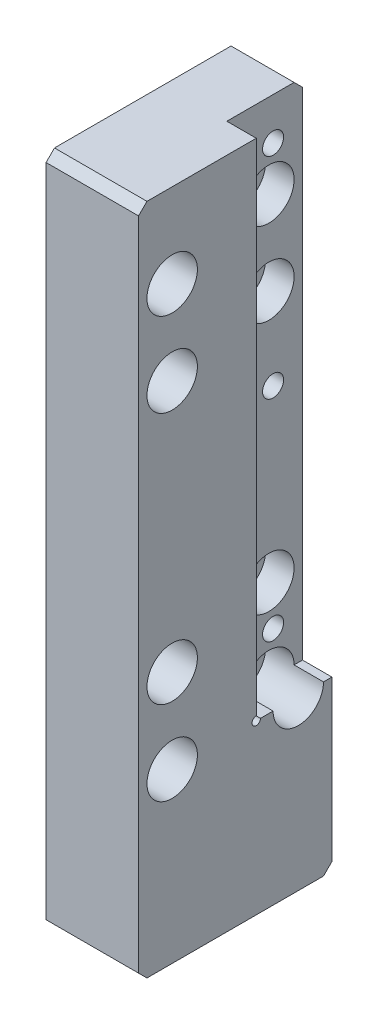
SolidWorks part; units mm, degrees
material "45#"
ref_plane "前基準面" through (0, 0, 0) normal (0, 0, 1) x (1, 0, 0)
ref_plane "上基準面" through (0, 0, 0) normal (0, 1, 0) x (1, 0, 0)
ref_plane "右基準面" through (0, 0, 0) normal (1, 0, 0) x (0, 0, -1)
sketch "草图1" plane through (0, 0, 0) normal (0, 1, 0) x (1, 0, 0)
  line L0 (0, 0) -> (0, 23)
  line L1 (0, 23) -> (11, 23)
  line L4 (11, 23) -> (11, 0)
  line L5 (11, 0) -> (0, 0)
  dimension "D2" = 11
  dimension "D3" = 23
extrude "凸台-拉伸1" add sketch "草图1" along normal blind 80
sketch "草图2" plane through (11, 0, 0) normal (1, 0, 0) x (0, 0, -1)
  line L1 (23, 80) -> (14, 80)
  line L2 (23, 80) -> (23, 20)
  line L3 (23, 20) -> (14.5, 20)
  line L4 (14, 80) -> (14, 20.5)
  arc A0 (14, 20.5) -> (14.5, 20) centre (14, 20) ccw
  dimension "D3" = 1
  dimension "D1" = 60
  dimension "D2" = 9
extrude "切除-拉伸1" cut sketch "草图2" against normal blind 3.5
hole_wizard "打孔尺寸(%根据)内六角圆柱头螺钉的类型2" positions "草图3" profile "草图4" counterbore size "M3" standard "GB" end condition through all
sketch "草图3" plane through (11, 0, 0) normal (1, 0, 0) x (0, 0, -1)
  line L0 (11.5, 0) -> (11.5, 103.8051) construction
  line L1 (0, 0) -> (23, 0) construction
  point P0 (4, 20)
  point P2 (4, 30)
  point P14 (19, 30)
  point P15 (19, 20)
  point P20 (4, 60)
  point P21 (4, 70)
  point P25 (19, 60) [skipped]
  point P26 (19, 70) [skipped]
  point P27 (19, 70)
  point P28 (19, 60)
  dimension "D1" = 15
  dimension "D2" = 20
  dimension "D3" = 10
  dimension "D5" = 40
  dimension "D4" = 2
sketch "草图4" plane through (11, 20, -4) normal (0, 1, 0) x (0, 0, -1)
  line L0 (0, 0) -> (0, 11)
  line L1 (0, 11) -> (1.7, 11)
  line L3 (1.7, 11) -> (1.7, 6.9)
  line L4 (1.7, 6.9) -> (3, 6.9)
  line L5 (3, 6.9) -> (3, 0)
  line L7 (3, 0) -> (0, 0)
  line L11 (0, -6.35) -> (0, 107.95) construction
  dimension "通孔孔直径" = 3.4
  dimension "通孔孔深度" = 11
  dimension "柱形沉头孔直径" = 6
  dimension "柱形沉头孔深度" = 6.9
hole_wizard "M5 螺纹孔1" positions "草图5" profile "草图6" tap size "M5" standard "GB"
sketch "草图5" plane through (0, 0, 0) normal (0, -1, 0) x (-1, 0, 0)
  line L4 (0, 11.5) -> (-11, 11.5) construction
  line L5 (0, 23) -> (0, 0) construction
  line L6 (-11, 0) -> (-11, 23) construction
  point P0 (-5.5, 11.5)
sketch "草图6" plane through (5.5, 0, -11.5) normal (1, 0, 0) x (0, 0, -1)
  line L0 (0, 0) -> (0, 13.6618)
  line L1 (0, 13.6618) -> (2.1, 12.4)
  line L2 (2.1, 12.4) -> (2.1, 0)
  line L5 (2.1, 0) -> (0, 0)
  line L10 (0, 13.6618) -> (-2.1, 12.4) construction
  line L11 (0, -6.35) -> (0, 107.95) construction
  dimension "螺纹孔钻头直径" = 4.2
  dimension "螺纹孔钻头深度" = 12.4
  dimension "导头角度" = 118
cosmetic thread "孔螺蚊线1" parameters "D1"=10, "D2"=5
hole_wizard "M3 螺纹孔1" positions "草图9" profile "草图10" tap size "M3" standard "GB" end condition through all
sketch "草图9" plane through (7.5, 0, 0) normal (1, 0, 0) x (0, 0, -1)
  line L0 (14.5, 20) -> (16, 20) construction
  line L1 (23, 20) -> (23, 80) construction
  point P0 (19.5, 25)
  point P8 (19.5, 50)
  point P9 (19.5, 75)
  dimension "D1" = 3
  dimension "D2" = 5
  dimension "D3" = 25
  dimension "D4" = 3.5
sketch "草图10" plane through (7.5, 25, -19.5) normal (0, 1, 0) x (0, 0, -1)
  line L0 (0, 0) -> (0, 7.5)
  line L1 (0, 7.5) -> (1.25, 7.5)
  line L2 (1.25, 7.5) -> (1.25, 0)
  line L5 (1.25, 0) -> (0, 0)
  line L11 (0, -6.35) -> (0, 107.95) construction
  dimension "通孔螺纹孔钻头直径" = 2.5
  dimension "通孔螺纹孔钻头深度" = 7.5
cosmetic thread "孔螺蚊线2" parameters "D2"=3
cosmetic thread "孔螺蚊线3" parameters "D2"=3
cosmetic thread "孔螺蚊线4" parameters "D2"=3
chamfer "倒角1" distance 1 angle 45 4 edges at (5.5, 0, -23) (5.5, 0, 0) (3.75, 80, -23) (5.5, 80, 0)
